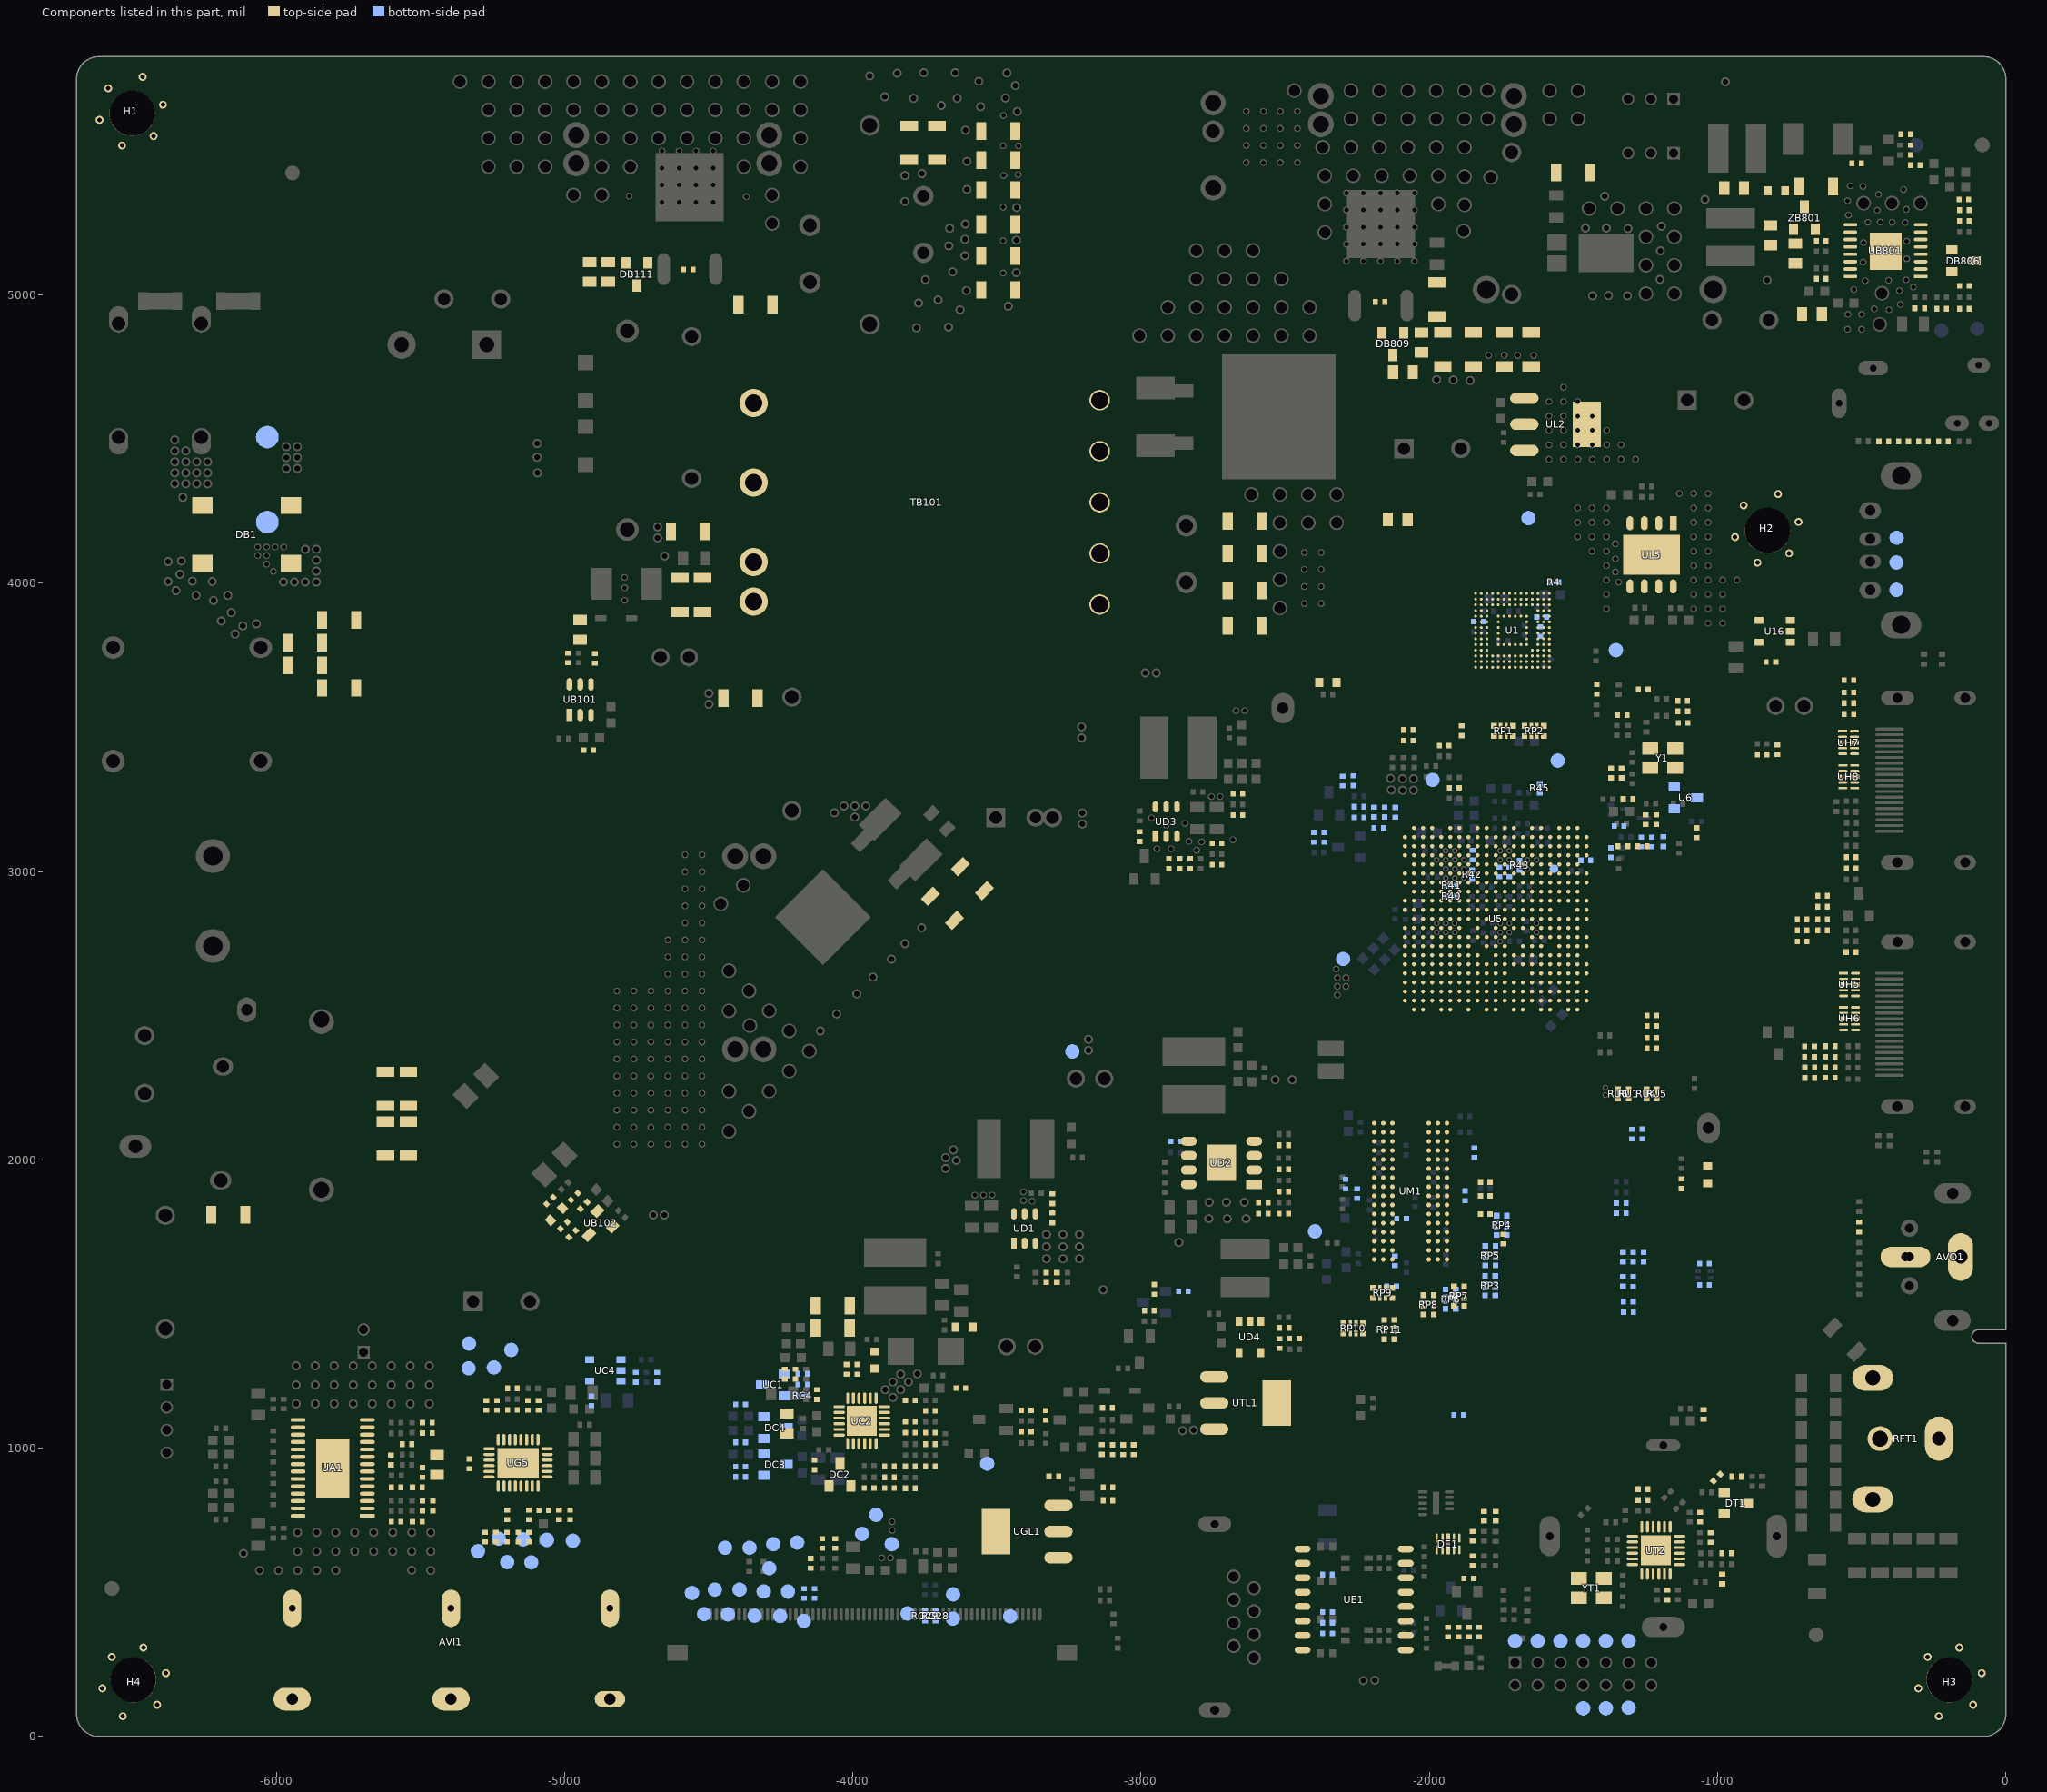
[diagram p0: the components of this part, seen from the top]
# Altium PCB MISC84395.PcbDoc (part 4 of 26)
Units mil, origin at the board's own origin, x right, y up, seen from the top; angles counter-clockwise.
Board outline 6692.91 x 5826.77 mil, 2 copper layers (TopLayer, BottomLayer), stack 61.855 mil thick; 951 components, 565 nets, 4374 pads, 1804 vias.
Unrouted connection lines stored in the file: 1.

## Components (designator, comment, footprint, x,y, rotation, side; value= is the part's Value field where it differs from the comment) (continued)
RB818 "0R3ohm-1206-±5%-1/4W" R1206 -1848,4810.94 r270 top
RB819 "0R3ohm-1206-±5%-1/4W" R1206 -1953.23,4810.94 r270 top
RB820 "0R3ohm-1206-±5%-1/4W" R1206 -1647,4811.06 r270 top
RB821 "NC/0R47ohm-1206-±1%-1/4W" R1206 -1740.77,4810.94 r270 top
RB822 "Thick film resistor,RES,1/16W,15Kohm,±1%,0402,SMD" R0402 -144.69,5294.13 r0 top
RB824 "NC/Thick film resistor,RES,1/8W,0ohm,±5%,0805,SMD" R0805 -817,5207 r90 top
RB825 "NC/Thick film resistor,RES,1/8W,0ohm,±5%,0805,SMD" R0805 -943,5370 r180 top
RB826 "NC/10ohm-1206-±5%-1/4W" R1206 -659,5376 r180 top
RB827 "510Kohm-0402-±1%-1/16W" R0402 -144.27,5031.32 r180 top
RB830 "Thick film resistor,RES,1/16W,3Kohm,±1%,0402,SMD" R0402 -314,5450 r180 top
RB832 "Thick film resistor,RES,1/16W,30Kohm,±1%,0402,SMD" R0402 -518,5456 r0 top
RB833 "Thick film resistor,RES,1/16W,2Kohm,±1%,0402,SMD" R0402 -330,5502.27 r270 top
RB834 "Thick film resistor,RES,1/16W,2Kohm,±1%,0402,SMD" R0402 -348,5557 r0 top
RB837 "Thick film resistor,RES,1/16W,12Kohm,±1%,0402,SMD" R0402 -145.73,5331 r0 top
RC1 "33ohm-0805-±5%-1/8W" R0805 -4229,1086 r90 top
RC2 "10Kohm-0402-±1%-1/16W" R0402 -4173.97,1221 r0 bottom
RC3 "2Kohm-0402-±1%-1/16W" R0402 -4173.97,1258 r180 bottom
RC4 "NC/0ohm-0402-PCB" R0402SC#1 -4173.97,1183 r0 bottom
RC5 "0ohm-0402-±5%-1/16W" R0402 -4022,1274 r270 top
RC6 "10Kohm-0402-±1%-1/16W" R0402 -3943,862 r0 top
RC7 "NC/12Kohm-0402-±1%-1/16W" R0402 -4199.24,1256.84 r90 top
RC8 "NC/0ohm-0402-±5%-1/16W" R0402 -4124,1186 r270 top
RC9 "NC/12Kohm-0402-±1%-1/16W" R0402 -4236.24,1256.84 r90 top
RC10 "100Kohm-0402-±1%-1/16W" R0402 -3873,862 r0 top
RC11 "Thick film resistor,RES,1/10W,22ohm,±5%,0603,SMD" R0603 -3923,1306 r270 top
RC12 "Thick film resistor,RES,1/16W,33Kohm,±1%,0402,SMD" R0402 -3801,1054 r0 top
RC13 "Thick film resistor,RES,1/16W,51Kohm,±5%,0402,SMD" R0402 -3801,1093 r0 top
RC14 "4R7ohm-0402-±5%-1/16W" R0402 -3731,1014 r0 top
RC15 "Thick film resistor,RES,1/16W,47Kohm,±1%,0402,SMD" R0402 -3731,1054 r0 top
RC16 "115Kohm-0402-±1%-1/16W" R0402 -3731,1130 r0 top
RC17 "10K5ohm-0402-±1%-1/16W" R0402 -3801,1166 r0 top
RC18 "47Kohm-0402-±5%-1/16W" R0402 -3625.27,1208.27 r180 top
RC19 "0ohm-0402-±5%-1/16W" R0402 -4389,900.19 r180 bottom
RC20 "NC/0ohm-0402-±5%-1/16W" R0402 -4389,936.19 r0 bottom
RC21 "62Kohm-0402-±1%-1/16W" R0402 -3731,937 r0 top
RC22 "7K5ohm-0402-±1%-1/16W" R0402 -3801,937 r0 top
RC23 "0ohm-0402-±5%-1/16W" R0402 -4389,1020.19 r0 bottom
RC24 "10Kohm-0402-±5%-1/16W" R0402 -4133,941.73 r270 top
RC25 "Thick film resistor,RES,1/16W,100Kohm,±1%,0402,SMD" R0402 -3801,861 r0 top
RC26 "4K7ohm-0402-±1%-1/16W" R0402 -3873,937 r180 top
RC27 "47Kohm-0402-±5%-1/16W" R0402 -4389,1152.19 r0 bottom
RC28 "Thick film resistor,RES,1/10W,22ohm,±5%,0603,SMD" R0603 -3614,1420 r0 top
RC29 "Thick film resistor,RES,1/16W,560ohm,±1%,0402,SMD" R0402 -3873,899 r0 top
RC31 "30Kohm-0402-±1%-1/16W" R0402 -4679,1245.73 r270 bottom
RC35 "10Kohm-0402-±1%-1/16W" R0402 -4753,1245.73 r90 bottom
RC36 "10ohm-0402-±5%-1/16W" R0402 -4906.73,1164.72 r270 bottom
RD1 "91Kohm-0402-±1%-1/16W" R0402 -3292,1592.27 r270 top
RD2 "100Kohm-0402-±5%-1/16W" R0402 -3308,1865 r270 top
RD3 "4K7ohm-0402-±5%-1/16W" R0402 -2503.73,1417.26 r0 top
RD4 "12Kohm-0402-±1%-1/16W" R0402 -3329,1592.27 r90 top
RD6 "10Kohm-0402-±5%-1/16W" R0402 -2575.73,1852 r180 top
RD7 "NC/18Kohm-0402-±1%-1/16W" R0402 -2505,1967 r0 top
RD8 "NC/" R0402 -2736.91,3097.93 r0 top
RD9 "NC/47Kohm-0402-±5%-1/16W" R0402 -3308,1799 r90 top
RD12 "15Kohm-0402-±1%-1/16W" R0402 -2505,1890 r0 top
RD13 "Thick film resistor,RES,1/16W,270Kohm,±1%,0402,SMD" R0402 -2903.26,3027.84 r90 top
RD15 "Thick film resistor,RES,1/16W,18.2Kohm,±1%,0402,SMD" R0402 -2737,3024.19 r180 top
RD16 "Thick film resistor,RES,1/16W,30Kohm,±1%,0402,SMD" R0402 -2829.26,3027.71 r90 top
RD17 "NC/?" R0402 -2866.26,3027.84 r90 top
RD18 "100ohm-0402-±5%-1/16W" R0402 -2505,2051 r0 top
RD19 "100ohm-0402-±5%-1/16W" R0402 -2880.73,2064 r180 bottom
RD24 "4K7ohm-0402-±5%-1/16W" R0402 -3005,3121 r90 top
RD25 "100Kohm-0402-±5%-1/16W" R0402 -2505,1814 r0 top
RD26 "100Kohm-0402-±5%-1/16W" R0402 -2664.29,3270.87 r0 top
RD27 "NC/1Mohm-0402-±5%-1/16W" R0402 -2664.29,3195.87 r0 top
RD28 "1Mohm-0402-±5%-1/16W" R0402 -2576,1814 r180 top
RD40 "4K7ohm-0402-±5%-1/16W" R0402 -1293.22,1578.04 r90 bottom
RD50 "62Kohm-0402-±1%-1/16W" R0402 -2468,1380.26 r0 top
RD51 "40K2ohm-0402-±1%-1/16W" R0402 -2520,1363 r270 top
RE1 "NC/75ohm-0402-±1%-1/16W" R0402 -2354,562 r180 bottom
RE2 "NC/75ohm-0402-±1%-1/16W" R0402 -2353,358 r180 bottom
RE3 "NC/75ohm-0402-±1%-1/16W" R0402 -2353,432 r180 bottom
RE4 "NC/75ohm-0402-±1%-1/16W" R0402 -2353,395 r180 bottom
RE11 "2R2ohm-0402-±1%-1/16W" R0402 -1228.65,2500.82 r0 top
RE12 "2R2ohm-0402-±1%-1/16W" R0402 -1228.65,2464.82 r0 top
RE13 "2R2ohm-0402-±1%-1/16W" R0402 -1228.65,2422.82 r0 top
RE14 "2R2ohm-0402-±1%-1/16W" R0402 -1228.65,2386.82 r0 top
RF1 "0ohm-0402-±5%-1/16W" R0402 -1333.65,3341.74 r270 top
RF2 "NC/1Mohm-0402-±5%-1/16W" R0402 -1369.65,3341.74 r270 top
RFT1 "RF header,RF JACK,H,IEC,T14.5,CH6.3,12.4×13.2×7.7mm,DIP,LHD-020 component,LHD" ANT-IEC14.5-H-4 -222,1033.46 r90 top locked
RG01 "NC/Thick film resistor,RES,1/16W,0ohm,±5%,0402,SMD" R0402 -3303,902 r180 top
RG1 "0ohm-0402-±5%-1/16W" R0402 -5090,1149 r270 top
RG02 "NC/Thick film resistor,RES,1/16W,0ohm,±5%,0402,SMD" R0402 -3115,864 r0 top
RG2 "0ohm-0402-±5%-1/16W" R0402 -5127,1149 r270 top
RG3 "Thick film resistor,RES,1/16W,0ohm,±5%,0402,SMD" R0402 -5330,946 r90 top
RG4 "Thick film resistor,RES,1/16W,0ohm,±5%,0402,SMD" R0402 -5271,1149 r270 top
RG5 "0ohm-0402-±5%-1/16W" R0402 -5072,785 r180 top
RG6 "NC/0ohm-0402-±5%-1/16W" R0402 -3985,1274 r90 top
RG7 "NC/Thick film resistor,RES,1/4W,3.3Kohm,±5%,1206,SMD" R1206 -4070.06,1494.76 r180 top
RG8 "NC/Thick film resistor,RES,1/4W,3.9Kohm,±5%,1206,SMD" R1206 -4070.06,1416.76 r180 top
RG9 "NC/Thick film resistor,RES,1/4W,3.3Kohm,±5%,1206,SMD" R1206 -4070,1417 r180 bottom
RG17 "33ohm-0402-±5%-1/16W" R0402 -4146,601 r270 top
RG18 "33ohm-0402-±5%-1/16W" R0402 -4061,670 r270 top
RG19 "33ohm-0402-±5%-1/16W" R0402 -4106,670 r270 top
RG24 "NC/10Kohm-0402-±5%-1/16W" R0402 -4133,496 r90 bottom
RG28 "NC/0ohm-0402-PCB" R0402SC#1 -3713,418 r90 bottom
RG29 "NC/0ohm-0402-PCB" R0402SC#1 -3749,418 r90 bottom
RG30 "4K7ohm-0402-±5%-1/16W" R0402 -4169,496.27 r270 bottom
RG79 "Thick film resistor,RES,1/16W,0ohm,±5%,0402,SMD" R0402 -5199,769 r90 top
RG80 "Thick film resistor,RES,1/16W,0ohm,±5%,0402,SMD" R0402 -5123.26,692 r90 top
RG81 "Thick film resistor,RES,1/16W,0ohm,±5%,0402,SMD" R0402 -5124,769 r90 top
RG82 "Thick film resistor,RES,1/16W,0ohm,±5%,0402,SMD" R0402 -4981,769 r90 top
RG84 "0ohm-0402-±5%-1/16W" R0402 -5019,769 r90 top
RG85 "Thick film resistor,RES,1/16W,0ohm,±5%,0402,SMD" R0402 -5160.51,691.5 r270 top
RG87 "Thick film resistor,RES,1/16W,0ohm,±5%,0402,SMD" R0402 -5199.51,691.5 r270 top
RG89 "Thick film resistor,RES,1/16W,0ohm,±5%,0402,SMD" R0402 -5238.51,691.5 r270 top
RG91 "Thick film resistor,RES,1/16W,0ohm,±5%,0402,SMD" R0402 -5275.51,691.5 r270 top
RH1 "1Kohm-0402-±5%-1/16W" R0402 -536.83,3050 r0 top
RH2 "10Kohm-0402-±5%-1/16W" R0402 -706.83,2834 r180 top
RH3 "10Kohm-0402-±5%-1/16W" R0402 -706.83,2796 r180 top
RH4 "10Kohm-0402-±5%-1/16W" R0402 -635.83,2878 r0 top
RH5 "10Kohm-0402-±5%-1/16W" R0402 -635.83,2834 r0 top
RH6 "22ohm-0402-±5%-1/16W" R0402 -635.83,2796 r180 top
RH7 "22ohm-0402-±5%-1/16W" R0402 -635.83,2916 r180 top
RH8 "33ohm-0402-±5%-1/16W" R0402 -536.83,3011 r0 top
RH9 "Thick film resistor,RES,1/16W,0ohm,±5%,0402,SMD" R0402 -537.27,2721 r0 top
RH10 "1Kohm-0402-±5%-1/16W" R0402 -680.83,2284.03 r180 top
RH11 "10Kohm-0402-±5%-1/16W" R0402 -681,2357.03 r180 top
RH12 "10Kohm-0402-±5%-1/16W" R0402 -681,2394.03 r0 top
RH13 "100ohm-0402-±5%-1/16W" R0402 -706.83,2758 r180 top
RH14 "10Kohm-0402-±5%-1/16W" R0402 -609.62,2321.24 r0 top
RH15 "10Kohm-0402-±5%-1/16W" R0402 -609.62,2285.24 r0 top
RH16 "22ohm-0402-±5%-1/16W" R0402 -609.62,2357.24 r180 top
RH17 "22ohm-0402-±5%-1/16W" R0402 -609.62,2394.24 r180 top
RH18 "33ohm-0402-±5%-1/16W" R0402 -680.83,2321.03 r180 top
RI1 "NC/0ohm-0402-±5%-1/16W" R0402 -509,1767.27 r270 top
RI4 "33ohm-0402-±5%-1/16W" R0402 -1328.65,3087.74 r0 top
RI5 "75ohm-0402-±1%-1/16W" R0402 -1261.65,3087.74 r180 top
RI7 "10Kohm-0402-±5%-1/16W" R0402 -1228.65,3102.74 r270 bottom
RI9 "12Kohm-0402-±1%-1/16W" R0402 -1264.65,3102.74 r270 bottom
RI11 "10Kohm-0402-±5%-1/16W" R0402 -1188.65,3103.74 r270 bottom
RI12 "12Kohm-0402-±1%-1/16W" R0402 -1341.65,3157.74 r180 bottom
RK1 "4K7ohm-0402-±1%-1/16W" R0402 -1309.46,1472 r180 bottom
RK2 "1Kohm-0402-±5%-1/16W" R0402 -1124.99,1917 r270 top
RK3 "10Kohm-0402-±5%-1/16W" R0402 -1899,362 r270 top
RK4 "100ohm-0402-±5%-1/16W" R0402 -1770,764 r270 top
RK5 "2K2ohm-0402-±1%-1/16W" R0402 -1863,362 r90 top
RK6 "NC/0ohm-0402-±5%-1/16W" R0402 -1935,362 r270 top
RK7 "10Kohm-0402-±5%-1/16W" R0402 -1864,548 r180 top
RK8 "10Kohm-0402-±5%-1/16W" R0402 -1850,610 r270 top
RK12 "4K7ohm-0402-±5%-1/16W" R0402 -1827,362 r270 top
RK14 "100ohm-0402-±5%-1/16W" R0402 -1811,764 r90 top
RL1 "NC/Thick film resistor,RES,1/16W,0ohm,±5%,0402,SMD" R0402 -2401,3119 r270 bottom
RL2 "NC/1Kohm-0402-±5%-1/16W" R0402 -2263,3314.74 r90 bottom
RL3 "NC/10Kohm-0402-±5%-1/16W" R0402 -2301,3314 r270 bottom
RL4 "NC/10Kohm-0402-±5%-1/16W" R0402 -2192,3206 r270 bottom
RL5 "100ohm-0402-±5%-1/16W" R0402 -2244,3225 r0 bottom
RL6 "100ohm-0402-±5%-1/16W" R0402 -845.83,3406 r0 top
RL7 "1Kohm-0402-±5%-1/16W" R0402 -2175,3152 r180 bottom
RL8 "4K7ohm-0402-±5%-1/16W" R0402 -792.83,3423 r270 top
RL9 "NC/Thick film resistor,RES,1/16W,0ohm,±5%,0402,SMD" R0402 -2244,3188 r0 bottom
RL10 "4K7ohm-0402-±5%-1/16W" R0402 -2155,3206 r90 bottom
RL11 "4K7ohm-0402-±5%-1/16W" R0402 -2118,3205.73 r90 bottom
RL12 "1Kohm-0402-±5%-1/16W" R0402 -2364,3119 r90 bottom
RM1 "4K7ohm-0402-±5%-1/16W" R0402 -2971.73,1477 r180 top
RM2 "4K7ohm-0402-±5%-1/16W" R0402 -3398,1131 r0 top
RM3 "NC/4K7ohm-0402-±5%-1/16W" R0402 -3331,1114 r90 top
RM4 "10Kohm-0402-±5%-1/16W" R0402 -1309.73,1509 r0 bottom
RM5 "100Kohm-0402-±5%-1/16W" R0402 -2954,1551 r90 top
RM7 "4K7ohm-0402-±5%-1/16W" R0402 -2853.27,1544 r180 bottom
RM8 "4K7ohm-0402-±5%-1/16W" R0402 -3026,995 r90 top
RM9 "10Kohm-0402-±5%-1/16W" R0402 -3062,995 r90 top
RM10 "2Kohm-0402-±1%-1/16W" R0402 -2119.47,1649.58 r90 bottom
RM11 "2Kohm-0402-±1%-1/16W" R0402 -1875.97,1875.82 r270 bottom
RM12 "Thick film resistor,RES,1/16W,100Kohm,±1%,0402,SMD" R0402 -3117,1140 r180 top
RM13 "NC/Thick film resistor,RES,1/16W,0ohm,±5%,0402,SMD" R0402 -1328.77,1578.27 r90 bottom
RM14 "Thick film resistor,RES,1/16W,0ohm,±5%,0402,SMD" R0402 -1898,1116 r0 bottom
RM15 "Thick film resistor,RES,1/16W,100Kohm,±1%,0402,SMD" R0402 -3398,1058 r180 top
RO4 "150ohm-0402-±1%-1/16W" R0402 -1334.73,1815.06 r0 bottom
RO45 "100ohm-0402-±5%-1/16W" R0402 -1334.73,1851.06 r180 bottom
RP1 "4*22ohm-0402-±5%-1/16W" RA0402 -1743.05,3487.34 r270 top
RP2 "4*22ohm-0402-±5%-1/16W" RA0402 -1636.21,3487.34 r270 top
RP3 "4*22ohm-0402-±5%-1/16W" RA0402 -1788.75,1563.72 r0 bottom
RP4 "4*22ohm-0402-±5%-1/16W" RA0402 -1748.85,1773.09 r0 bottom
RP5 "4*22ohm-0402-±5%-1/16W" RA0402 -1788.67,1667.28 r0 bottom
RP6 "4*22ohm-0402-±5%-1/16W" RA0402 -1925.97,1517.19 r0 bottom
RP7 "4*22ohm-0402-±5%-1/16W" RA0402 -1896.94,1527.03 r0 top
RP8 "4*22ohm-0402-±5%-1/16W" RA0402 -2002.74,1497.5 r0 top
RP9 "4*22ohm-0402-±5%-1/16W" RA0402 -2161.83,1538.35 r270 top
RP10 "4*22ohm-0402-±5%-1/16W" RA0402 -2264.55,1415.32 r270 top
RP11 "4*22ohm-0402-±5%-1/16W" RA0402 -2139.04,1411.38 r0 top
RS1 "Ferrite bead,BEAD,120ohm,0603,2000mA,SMD,TP,HCB1608KF-121T20,TAI-TECH" R0603 -2352,3656 r180 top
RS2 "Ferrite bead,BEAD,120ohm,0603,2000mA,SMD,TP,HCB1608KF-121T20,TAI-TECH" R0603 -1034,1949 r270 top
RT1 "750Kohm-0402-±5%-1/16W" R0402 -1174.21,491.19 r270 top
RT2 "100ohm-0402-±5%-1/16W" R0402 -1121,3592.13 r180 top
RT4 "100ohm-0402-±5%-1/16W" R0402 -1120.73,3556 r180 top
RT5 "100ohm-0402-±5%-1/16W" L0402 -1259,858 r180 top
RT6 "100ohm-0402-±5%-1/16W" R0402 -1061,761 r90 top
RT7 "10Kohm-0402-±5%-1/16W" R0402 -1419,3633 r270 top
RT9 "100ohm-0402-±5%-1/16W" R0402 -1003,898 r45 top
RT10 "100ohm-0402-±5%-1/16W" L0402 -1259,820 r180 top
RT14 "NC/?" R0402 -1330.65,3542.74 r0 top
RT34 "4K7ohm-0402-±5%-1/16W" R0402 -1328.82,1662.26 r270 bottom
RT36 "4K7ohm-0402-±5%-1/16W" R0402 -1292.83,1662.26 r90 bottom
RT39 "4K7ohm-0402-±5%-1/16W" R0402 -1257.83,3632 r180 top
RT40 "4K7ohm-0402-±5%-1/16W" R0402 -1120,3516 r0 top
RU1 "NC/0ohm-0402-PCB" R0402SC#1 -1308.83,2229 r90 top
RU2 "0ohm-0402-±5%-1/16W" R0402 -1046,1566 r180 bottom
RU3 "10Kohm-0402-±5%-1/16W" R0402 -544.83,3621 r180 top
RU4 "NC/0ohm-0402-PCB" R0402SC#1 -1246.83,2229 r90 top
RU5 "NC/0ohm-0402-PCB" R0402SC#1 -1210.83,2229 r90 top
RU6 "NC/0ohm-0402-PCB" R0402SC#1 -1344.83,2229 r90 top
RU7 "NC/4K7ohm-0402-±5%-1/16W" R0402 -544.83,3664 r180 top
RU8 "0ohm-0402-±5%-1/16W" R0402 -1046,1640 r180 bottom
RU9 "10Kohm-0402-±5%-1/16W" R0402 -544.83,3584 r180 top
RU10 "NC/10Kohm-0402-±5%-1/16W" R0402 -815,3727 r180 top
RU12 "NC/4K7ohm-0402-±5%-1/16W" R0402 -544.83,3546 r180 top
RV15 "4K7ohm-0402-±5%-1/16W" R0402 -354.83,4492.16 r0 top
RV16 "100ohm-0402-±5%-1/16W" R0402 -423.83,4492.16 r180 top
RV17 "4K7ohm-0402-±5%-1/16W" R0402 -285.83,4492 r180 top
RV18 "100ohm-0402-±5%-1/16W" R0402 -216.83,4492 r180 top
RW1 "Thick film resistor,RES,1/16W,56Kohm,±1%,0402,SMD" R0402 -5181,1208 r180 top
RW2 "Thick film resistor,RES,1/16W,33Kohm,±1%,0402,SMD" R0402 -5181,1133 r180 top
RW3 "NC/?" R0402 -5234,1149 r270 top
S/N1 "Barcode" Barcode -3116,2745 r0 bottom
S/N2 "Barcode" Barcode -4647,2486 r270 top
STV "TEST" TP#2 -5061.26,682 r90 bottom
STV_IN "TEST" TP#2 -5185,1341 r90 bottom
TB101 "Transformer,EQ2612,450uH,0.26×2P,35Ts,H14.5MAX,SYEQ2612-T004,DIP,SQ" T/EQ2512*11 -3850.22,4280.51 r0 top locked
TCON_DVDD "TEST" TP#1 -3919,769 r180 bottom
TP1 "TEST" TP#1 -3653,409 r90 bottom
TP-TDT "NC/" TP-TDT -6031,4359.64 r90 bottom
U1 "eMMC FLASH chip,IC EMMC FLASH,4GB,32Gb,MLC,FBGA153,SMD,KLM4G1FETE-B041,Samsung" BGA153/0.5-1 -1711.87,3836.56 r180 top locked
U5 "Customer-supplied main chip,IC Main Chip,SMD,MSD6A346ATT-8-XZ,COMPANY_A-QD,MTK" BGA406/0.8 -1769.97,2836.08 r180 top locked
U6 "NC/SGM810-SXN3L" SO-23-1 -1110,3256 r90 bottom
U16 "Current-limit switch,IC OCP,1.0A,5.5V,SOT23-5,SMD,APL3551CBI-TRG,ANPEC" SOT-23-5 -801.83,3833 r90 top
UA1 "Audio amplifier,IC Audio AMP,Class D,2X8W@12V@8ohm,E-TSSOP-28L,SMD,AD52050B-26QG28NRR,ESMT" SOP28/0.65-7 -5804.15,931.94 r180 top locked
UB101 "PWM controller,IC PWM Controller,65KHz,SOT-26,SMD,SR12 GL,Leadtrend" SOT-26 -4945.49,3596.15 r180 top
UB102 "Regulator,IC Regulator,2.50V,0.4%,SOT-23,SMD,BR431M-A,Blue Rocket" SOT-23-RAK -4887.77,1767.2 r135 top
UB801 "PWM controller,IC PWM Controller,200KHz,SOP-16,SMD,MP3398AGF-Z,MPS" TSSOP16/0.65-3 -417.58,5151.39 r180 top
UC1 "AZ431AN-ATRE1(BCD)" SO-23-1 -4276.97,1220 r270 bottom
UC2 "Tcon driver chip,IC Tcon Driver,VQFN-24L,SMD,ANX6732AAQX,ANAX" QFN24/0.5-5 -3968.74,1094.92 r0 top locked
UC4 "Op amp,IC OP Amplifier,1 channel,18MHz,TSOT23-5,SMD,ANX7003AAK,ANAX" SOT-23-5 -4859,1269.73 r270 bottom
UD1 "DC-DC chip,IC DC-DC,Syn,3A,18V,500kHz,SOT23-6,SMD,SY8113IADC,Silergy" TSOT23-6 -3404,1762 r90 top
UD2 "Customer-supplied DC-DC chip,IC DCDC,SMD,MSH6110A,COMPANY_A-QD,MTK" SOP8/1.27 -2721,1990 r180 top
UD3 "DC-DC chip,IC DC-DC,Syn,3A,18V,500kHz,SOT23-6,SMD,SY8113IADC,Silergy" TSOT23-6 -2913,3173.19 r90 top
UD4 "DC-DC chip,IC DCDC,Syn,1A,5.5V,1.5MHz,SOT23-5,SMD,SY8088IAAC,Silergy" SOT-23-5 -2622.21,1386.29 r180 top
UE1 "NC/Network transformer,Net Transformer,350uH,0.09×1P,H6.0MAX,B1601S,SMD,DDY" SOP16/1.27-2 -2261.1,475.71 r180 top locked
UG5 "LCD level-shift chip,IC LCD Driver,TQFN4X5-28,SMD,KD595EKL1U,GMT" QFN28/0.5-5 -5161,949 r270 top locked
UGL1 "NC/LC1117CLTR33" SOT-223 -3395,711 r90 top locked
UH5 "NC/TVS diode,DIO ESD,0.4pF,19V,DFN2510-10L,SMD,ESD5304D-10/TR,Willsemi" RCL0524P -542.34,2608.02 r270 top
UH6 "NC/TVS diode,DIO ESD,0.4pF,19V,DFN2510-10L,SMD,ESD5304D-10/TR,Willsemi" RCL0524P -542.34,2489.91 r270 top
UH7 "NC/TVS diode,DIO ESD,0.4pF,19V,DFN2510-10L,SMD,ESD5304D-10/TR,Willsemi" RCL0524P -545.84,3447.78 r270 top
UH8 "NC/TVS diode,DIO ESD,0.4pF,19V,DFN2510-10L,SMD,ESD5304D-10/TR,Willsemi" RCL0524P -545.34,3328.78 r270 top
UL2 "LC1117CLTR33" SOT-223 -1562.27,4551 r270 top
UL5 "LDO chip,IC LDO,1A,1.8&3.3V,12V,SOP-8,SMD,SA1118B-1833,SL" SOP8/1.27-3 -1229.2,4098.55 r270 top
UM1 "DDR chip,IC DDR3,DDR3,2133M,16bit,512MB,4Gb,FBGA96,SMD,K4B4G1646E-BCNB,Samsung" BGA96/0.8-1 -2065.24,1891.2 r0 top locked
USB_5V "TEST" TP#2 -380,3977 r90 bottom
UT2 "MxL661" QFN24/0.5-1 -1213.89,645.47 r180 top locked
UTL1 "NC/LC1117CLTR33" SOT-223 -2638,1157 r270 top
VCC_PANEL "TEST" TP#1 -3534,946 r180 bottom
VDD1 "TEST" TP#2 -4971,679 r180 bottom
VDD2 "TEST" TP#1 -3652,493 r180 bottom
VREF "TEST" TP#1 -3968,703 r180 bottom
VSS1 "TEST" TP#1 -4558,498 r180 bottom
WIFI_RST "TEST" TP#2 -1466.48,98 r90 bottom
XXXXXX "PCB_TIME" PCB_TIME -1694,1120 r90 top
XXXXXXXXXXXXXXXX "PCB_NAME" PCB_NAME -1755.31,1282.16 r90 top
Y1 "Passive crystal oscillator,SPXO,24MHz,±10ppm,12pF,SMD3225-metal case,SMD,JWT" XTAL-S-3 -1191.34,3394.2 r0 top
YT1 "Passive standard-package crystal oscillator,SPXO,16MHz,±10ppm,9pF,SMD3225,SMD,CF4016M00009T2115013,JWT" XTAL-S-3 -1438,515 r180 top
ZB801 "NC/Zener diode,DIO ZEN,15V,300mW,SOT-23,SMD,BZX84C15,BLUE ROCKET" SO-23 -699,5268 r180 top
用于U5上 "Thermal grease,0.05g,other,white,NULL" "Heat-Shrinkable Tube" 1655.21,5847.5 r270 top

## Footprints (in the part's own frame and the unit in brackets; to place one, negate y for a bottom-side part, rotate by r counter-clockwise, add the part's x,y. Pads: shape width x height; smd on the part's side, far side on the other; paste and mask are expansions set on the pad)
AI_GRIPPER_V [mm] "3D shape for vertical type AI equipment  (AI爪子)"
  round 1.5 on Mech5: 0(0,-2.5) 1(0,0) 2(0,2.5)
  body extent -29.13,-4.7 2.5,4.7, height 54.74
ANT-IEC14.5-H-4 [mm] "联宏达；13.2×12.4×7.7mm LHD-020 中心高度6.3mm 160323(18.03.09更新脚距）,向内扩宽丝印,0703_2018（18.08.29 更新短槽孔）"
  oval 2.5x3.8 on Top Overlay paste-4 mask-4: 0(-5.35,6.1) 0(5.35,6.1)
  round 2.4 on Top Overlay: 0(0,5.45)
  oval 4.1x2.7 on Top Overlay paste-4 mask-4: 0(0,0.25)
  round 2.2 hole 1.4: 1(0,5.45)
  oval 2.3x3.6 hole 1.3 slot 2.6 at 90 deg: 2(-5.35,6.1) 4(5.35,6.1)
  oval 3.9x2.5 hole 1.2 slot 2.6 at 0 deg: 3(0,0.25)
  KeepOutLayer pour cut-out: 0,3.95 -0.574,4.064 -1.061,4.389 -1.386,4.876 -1.5,5.45 -1.5,5.45 -1.386,6.024 -1.061,6.511 -0.574,6.836 0,6.95 0,6.95 0.574,6.836 1.061,6.511 1.386,6.024 1.5,5.45 1.5,5.45 1.386,4.876 1.061,4.389 0.574,4.064 0,3.95
  silkscreen extent -6.3,0 6.3,7.9, body extent -7.55,-35.2 7.55,7.7, height 13.76
ASSE4.0C-3 [mm] "定位孔(顶底层上锡)(17.12.09更新过孔位置）18.11.22 更新paste形状为扇形。"
  round 4 hole 4 unplated mask+0: 0(0,0)
  round 0.7 hole 0.4: 1(-2.72,-0.754) 2(-1.893,2.011) 3(0.891,2.84) 4(2.873,0.584) 5(2.105,-2.203) 6(-0.924,-3.213)
  KeepOutLayer pour cut-out: 0,-2.3 -0.88,-2.125 -1.626,-1.626 -2.125,-0.88 -2.3,0 -2.3,0 -2.125,0.88 -1.626,1.626 -0.88,2.125 0,2.3 0,2.3 0.88,2.125 1.626,1.626 2.125,0.88 2.3,0 2.3,0 2.125,-0.88 1.626,-1.626 0.88,-2.125 0,-2.3
AV1-H-1 [mm] "百汇 AV-8.4-5    出口中心高度为6.5MM"
  rrect50% 1.9x1.8 on Keep-Out: 0(-4.25,0.9) 0(4.25,0.9)
  oval 2x4.6 on Top Overlay: 0(0.002,8.85)
  oval 4.4x2.4 on Top Overlay: 0(0.002,4)
  oval 1.8x4.4 hole 0.8 slot 3.4 at 90 deg: 1(0.002,8.85)
  oval 4.2x2.2 hole 1.2 slot 3.2 at 0 deg: 2(0.002,4)
  silkscreen extent -5,0 5,10.2, body extent -5,-9.53 5,9.97, height 11
AV3-V14-1 [mm] "百汇AV3-8.4-46A 立式14间距，（17.03.20更新3D和前视图位置）"
  oval 3.5x2.2 on Top Overlay: 0(-14,-5.2) 0(0,-5.2) 0(14,-5.2)
  oval 1.8x3.5 on Top Overlay: 0(-14,2.8) 0(0,2.8) 0(14,2.8)
  oval 4.1x2.1 on Keep-Out paste-4 mask-4: 0(-7,4.9) 0(7,-4.9)
  oval 1.6x3.3 hole 0.6 slot 2.3 at 90 deg: 1(-14,2.8) 3(0,2.8) 5(14,2.8)
  oval 3.3x2 hole 1 slot 2.3 at 0 deg: 2(-14,-5.2) 4(0,-5.2)
  oval 2.69x1.416 / inner oval 3.3x2 / far side oval 3.3x2 hole 1 slot 2.3 at 0 deg: 6(14,-5.2)
  silkscreen extent -20.5,-6.5 20.5,6.5, body extent -20.5,-6.5 20.5,6.5, height 19.2
B/YBS3010A [mm] "YJ,YBS3010A,18.04.17"
  rect 1.5x1.8 smd: 1(2.55,3.9) 2(2.55,-3.9) 3(-2.55,-3.9) 4(-2.55,3.9)
  silkscreen extent -3.35,-3.7 3.35,5.74, body extent -3.35,-3.7 3.35,3.7, height 1.5
Barcode [mm] "(18.12.17 更新为白油）"
  round 0.3 on Mech2: 0(0,0)
  silkscreen extent -15,-4 15,4
BGA96/0.8-1 [mm] "SKhynix；4GB DDR3 SDRAM　 9.4*13／NANYA　SDRAM B-Die　10*13兼容"
  round 0.4 smd: A1(-3.2,6) A2(-2.4,6) A3(-1.6,6) A7(1.6,6) A8(2.4,6) A9(3.2,6) B1(-3.2,5.2) B2(-2.4,5.2) B3(-1.6,5.2) B7(1.6,5.2) B8(2.4,5.2) B9(3.2,5.2) C1(-3.2,4.4) C2(-2.4,4.4) C3(-1.6,4.4) C7(1.6,4.4) C8(2.4,4.4) C9(3.2,4.4) D1(-3.2,3.6) D2(-2.4,3.6) D3(-1.6,3.6) D7(1.6,3.6) D8(2.4,3.6) D9(3.2,3.6) E1(-3.2,2.8) E2(-2.4,2.8) E3(-1.6,2.8) E7(1.6,2.8) E8(2.4,2.8) E9(3.2,2.8) F1(-3.2,2) F2(-2.4,2) F3(-1.6,2) F7(1.6,2) F8(2.4,2) F9(3.2,2) G1(-3.2,1.2) G2(-2.4,1.2) G3(-1.6,1.2) G7(1.6,1.2) G8(2.4,1.2) G9(3.2,1.2) H1(-3.2,0.4) H2(-2.4,0.4) H3(-1.6,0.4) H7(1.6,0.4) H8(2.4,0.4) H9(3.2,0.4) J1(-3.2,-0.4) J2(-2.4,-0.4) J3(-1.6,-0.4) J7(1.6,-0.4) J8(2.4,-0.4) J9(3.2,-0.4) K1(-3.2,-1.2) K2(-2.4,-1.2) K3(-1.6,-1.2) K7(1.6,-1.2) K8(2.4,-1.2) K9(3.2,-1.2) L1(-3.2,-2) L2(-2.4,-2) L3(-1.6,-2) L7(1.6,-2) L8(2.4,-2) L9(3.2,-2) M1(-3.2,-2.8) M2(-2.4,-2.8) M3(-1.6,-2.8) M7(1.6,-2.8) M8(2.4,-2.8) M9(3.2,-2.8) N1(-3.2,-3.6) N2(-2.4,-3.6) N3(-1.6,-3.6) N7(1.6,-3.6) N8(2.4,-3.6) N9(3.2,-3.6) P1(-3.2,-4.4) P2(-2.4,-4.4) P3(-1.6,-4.4) P7(1.6,-4.4) P8(2.4,-4.4) P9(3.2,-4.4) R1(-3.2,-5.2) R2(-2.4,-5.2) R3(-1.6,-5.2) R7(1.6,-5.2) R8(2.4,-5.2) R9(3.2,-5.2) T1(-3.2,-6) T2(-2.4,-6) T3(-1.6,-6) T7(1.6,-6) T8(2.4,-6) T9(3.2,-6)
  silkscreen extent -5.59,-6.7 5.05,7.84, body extent -5.05,-6.55 5.05,6.55, height 1.2
BGA153/0.5-1 [mm] "SANDISK;iNAND/THGBMBG5D1KBAIT(10*11);14.05.16修改;170408兼容1.2mm高度"
  round 0.25 smd mask+0.051: A1(-3.25,3.25) A2(-2.75,3.25) A3(-2.25,3.25) A4(-1.75,3.25) A5(-1.25,3.25) A6(-0.75,3.25) A7(-0.25,3.25) A8(0.25,3.25) A9(0.75,3.25) A10(1.25,3.25) A11(1.75,3.25) A12(2.25,3.25) A13(2.75,3.25) A14(3.25,3.25) B1(-3.25,2.75) B2(-2.75,2.75) B3(-2.25,2.75) B4(-1.75,2.75) B5(-1.25,2.75) B6(-0.75,2.75) B7(-0.25,2.75) B8(0.25,2.75) B9(0.75,2.75) B10(1.25,2.75) B11(1.75,2.75) B12(2.25,2.75) B13(2.75,2.75) B14(3.25,2.75) C1(-3.25,2.25) C2(-2.75,2.25) C3(-2.25,2.25) C4(-1.75,2.25) C5(-1.25,2.25) C6(-0.75,2.25) C7(-0.25,2.25) C8(0.25,2.25) C9(0.75,2.25) C10(1.25,2.25) C11(1.75,2.25) C12(2.25,2.25) C13(2.75,2.25) C14(3.25,2.25) D1(-3.25,1.75) D2(-2.75,1.75) D3(-2.25,1.75) D4(-1.75,1.75) D12(2.25,1.75) D13(2.75,1.75) D14(3.25,1.75) E1(-3.25,1.25) E2(-2.75,1.25) E3(-2.25,1.25) E5(-1.25,1.25) E6(-0.75,1.25) E7(-0.25,1.25) E8(0.25,1.25) E9(0.75,1.25) E10(1.25,1.25) E12(2.25,1.25) E13(2.75,1.25) E14(3.25,1.25) F1(-3.25,0.75) F2(-2.75,0.75) F3(-2.25,0.75) F5(-1.25,0.75) F10(1.25,0.75) F12(2.25,0.75) F13(2.75,0.75) F14(3.25,0.75) G1(-3.25,0.25) G2(-2.75,0.25) G3(-2.25,0.25) G5(-1.25,0.25) G10(1.25,0.25) G12(2.25,0.25) G13(2.75,0.25) G14(3.25,0.25) H1(-3.25,-0.25) H2(-2.75,-0.25) H3(-2.25,-0.25) H5(-1.25,-0.25) H10(1.25,-0.25) H12(2.25,-0.25) H13(2.75,-0.25) H14(3.25,-0.25) J1(-3.25,-0.75) J2(-2.75,-0.75) J3(-2.25,-0.75) J5(-1.25,-0.75) J10(1.25,-0.75) J12(2.25,-0.75) J13(2.75,-0.75) J14(3.25,-0.75) K1(-3.25,-1.25) K2(-2.75,-1.25) K3(-2.25,-1.25) K5(-1.25,-1.25) K6(-0.75,-1.25) K7(-0.25,-1.25) K8(0.25,-1.25) K9(0.75,-1.25) K10(1.25,-1.25) K12(2.25,-1.25) K13(2.75,-1.25) K14(3.25,-1.25) L1(-3.25,-1.75) L2(-2.75,-1.75) L3(-2.25,-1.75) L12(2.25,-1.75) L13(2.75,-1.75) L14(3.25,-1.75) M1(-3.25,-2.25) M2(-2.75,-2.25) M3(-2.25,-2.25) M4(-1.75,-2.25) M5(-1.25,-2.25) M6(-0.75,-2.25) M7(-0.25,-2.25) M8(0.25,-2.25) M9(0.75,-2.25) M10(1.25,-2.25) M11(1.75,-2.25) M12(2.25,-2.25) M13(2.75,-2.25) M14(3.25,-2.25) N1(-3.25,-2.75) N2(-2.75,-2.75) N3(-2.25,-2.75) N4(-1.75,-2.75) N5(-1.25,-2.75) N6(-0.75,-2.75) N7(-0.25,-2.75) N8(0.25,-2.75) N9(0.75,-2.75) N10(1.25,-2.75) N11(1.75,-2.75) N12(2.25,-2.75) N13(2.75,-2.75) N14(3.25,-2.75) P1(-3.25,-3.25) P2(-2.75,-3.25) P3(-2.25,-3.25) P4(-1.75,-3.25) P5(-1.25,-3.25) P6(-0.75,-3.25) P7(-0.25,-3.25) P8(0.25,-3.25) P9(0.75,-3.25) P10(1.25,-3.25) P11(1.75,-3.25) P12(2.25,-3.25) P13(2.75,-3.25) P14(3.25,-3.25)
  silkscreen extent -6.43,-6.55 5.8,7.55